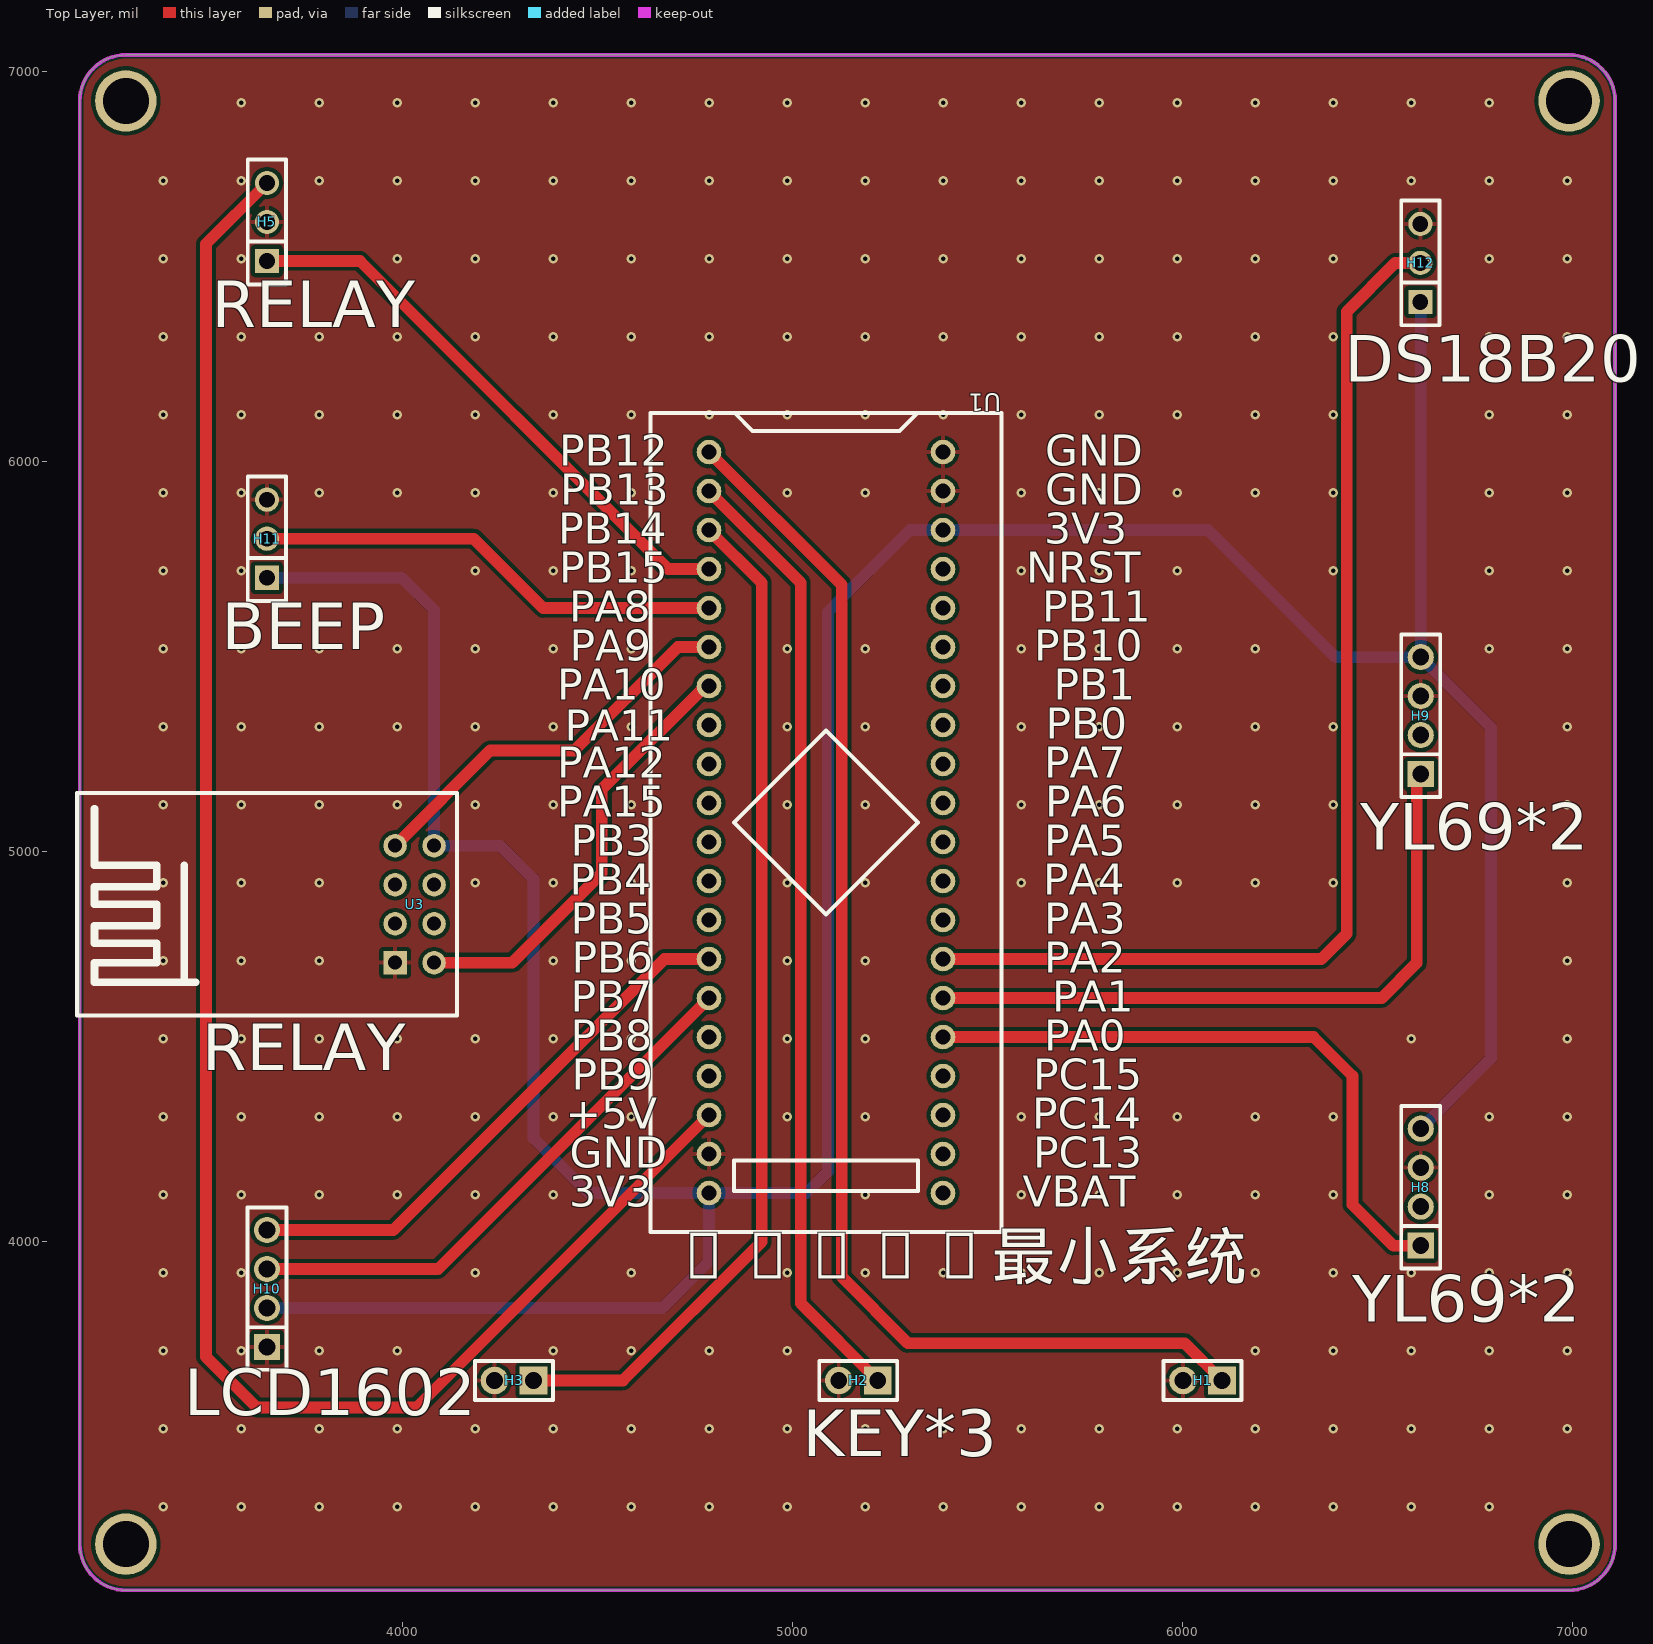
[diagram p0: Top Layer view]
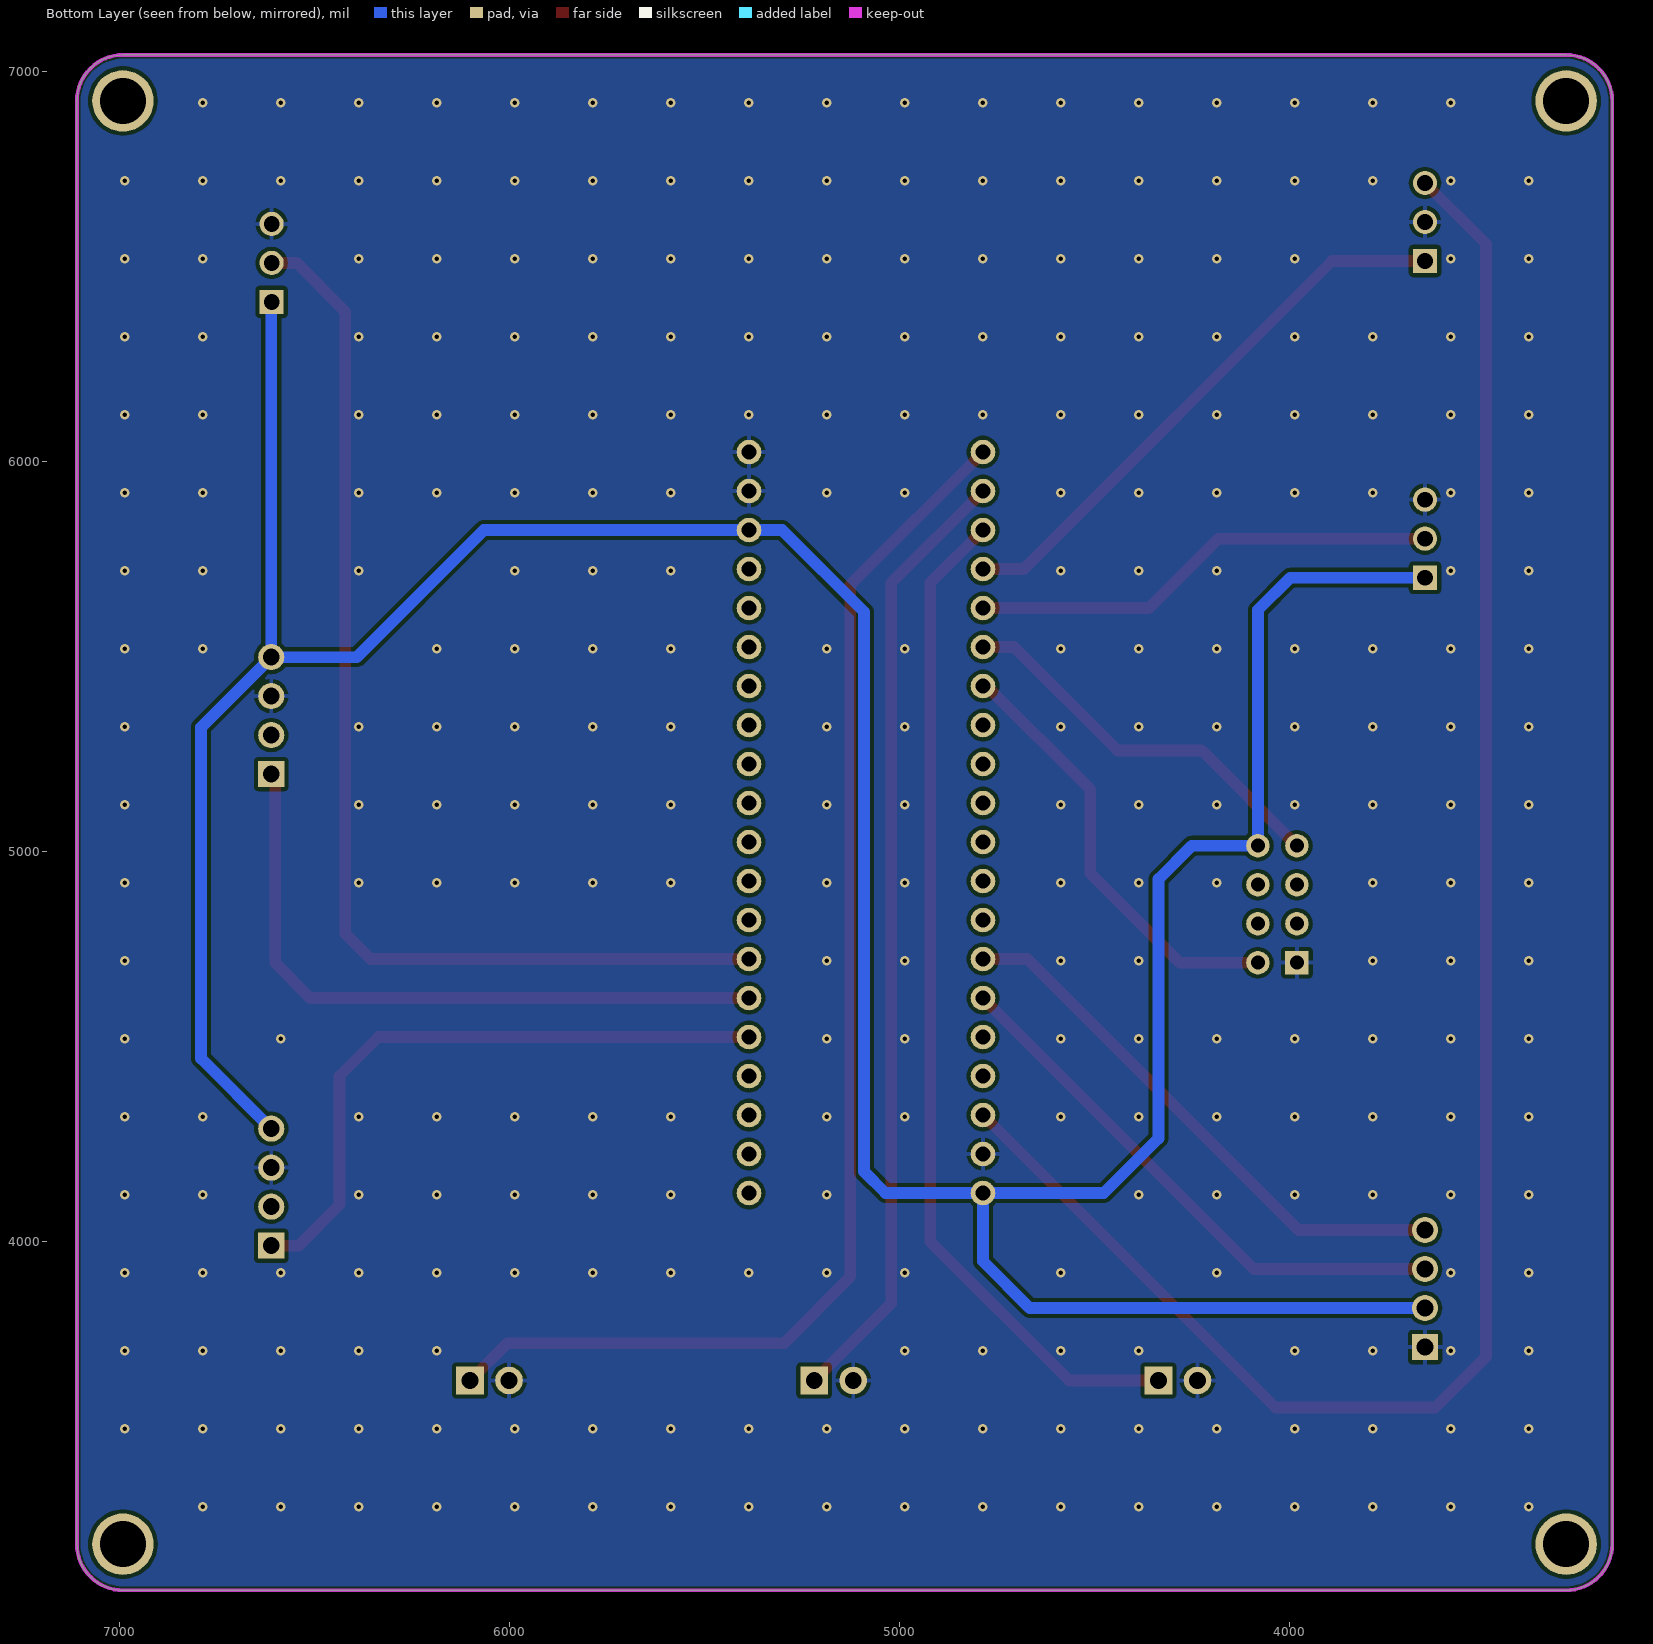
[diagram p1: Bottom Layer view, seen from below]
# Altium PCB MISC51268.pcbdoc
Units mil, origin at the board's own origin, x right, y up, seen from the top; angles counter-clockwise.
Board outline 3937.01 x 3937.01 mil, 2 copper layers (Top Layer, Bottom Layer), stack 62.206 mil thick; 11 components, 37 nets, 79 pads, 289 vias.

## Layer stack, top to bottom
Top Solder Mask Layer: solder mask 0.394, Dk 3.3
Top Layer: signal copper 1.379
Dielectric1: surface 59.449, FR4, Dk 4.5
Bottom Layer: signal copper 1.378
Bottom Solder Mask Layer: solder mask 0.394, Dk 3.3

## Board outline
6990.39,3106.5 ccw(c6990.39,3224.61) 7108.5,3224.61 7108.5,6925.39 ccw(c6990.39,6925.39) 6990.39,7043.5 3289.61,7043.5 ccw(c3289.61,6925.39) 3171.5,6925.39 3171.5,3224.61 ccw(c3289.61,3224.61) 3289.61,3106.5

## Design rules (kind name [scope] priority, off if disabled: settings)
BoardOutlineClearance copperThickness2oz_1 [All] p2 off: genericclearance=7.99 ignorepadtopadclearanceinfootprint=FALSE except(0: Arc-SplitContinuation Track-SplitContinuation SMDPad-SplitContinuation THPad-SplitContinuation Via-SplitContinuation Fill-SplitContinuation Region-SplitContinuation Poly-SplitContinuation Text-SplitContinuation Hole-SplitContinuation; 5.98: Arc-CutoutEdge Track-CutoutEdge SMDPad-CutoutEdge THPad-CutoutEdge Via-CutoutEdge Text-CutoutEdge; 6.89: Hole-OutlineEdge Hole-CutoutEdge; 10: Poly-OutlineEdge Poly-CutoutEdge; 11.81: Arc-OutlineEdge Track-OutlineEdge SMDPad-OutlineEdge THPad-OutlineEdge Via-OutlineEdge Fill-OutlineEdge Region-OutlineEdge Text-OutlineEdge Fill-CutoutEdge Region-CutoutEdge)
BoardOutlineClearance Plane_innerPlane_1 [All] p4 off: genericclearance=4.02 ignorepadtopadclearanceinfootprint=FALSE except(0: Arc-SplitContinuation Track-SplitContinuation SMDPad-SplitContinuation THPad-SplitContinuation Via-SplitContinuation Fill-SplitContinuation Region-SplitContinuation Poly-SplitContinuation Text-SplitContinuation Hole-SplitContinuation; 5.98: Arc-CutoutEdge Track-CutoutEdge SMDPad-CutoutEdge THPad-CutoutEdge Via-CutoutEdge Text-CutoutEdge; 6.89: Hole-OutlineEdge Hole-CutoutEdge; 10: Poly-OutlineEdge Poly-CutoutEdge; 11.81: Arc-OutlineEdge Track-OutlineEdge SMDPad-OutlineEdge THPad-OutlineEdge Via-OutlineEdge Fill-OutlineEdge Region-OutlineEdge Text-OutlineEdge Fill-CutoutEdge Region-CutoutEdge)
BoardOutlineClearance Copper_copperRegion_1 [All] p6 off: genericclearance=4.02 ignorepadtopadclearanceinfootprint=FALSE except(0: Arc-SplitContinuation Track-SplitContinuation SMDPad-SplitContinuation THPad-SplitContinuation Via-SplitContinuation Fill-SplitContinuation Region-SplitContinuation Poly-SplitContinuation Text-SplitContinuation Hole-SplitContinuation; 5.98: Arc-CutoutEdge Track-CutoutEdge SMDPad-CutoutEdge THPad-CutoutEdge Via-CutoutEdge Text-CutoutEdge; 6.89: Hole-OutlineEdge Hole-CutoutEdge; 10: Poly-OutlineEdge Poly-CutoutEdge; 11.81: Arc-OutlineEdge Track-OutlineEdge SMDPad-OutlineEdge THPad-OutlineEdge Via-OutlineEdge Fill-OutlineEdge Region-OutlineEdge Text-OutlineEdge Fill-CutoutEdge Region-CutoutEdge)
BoardOutlineClearance copperThickness1oz_1 [All] p8: genericclearance=4.02 ignorepadtopadclearanceinfootprint=FALSE except(0: Arc-SplitContinuation Track-SplitContinuation SMDPad-SplitContinuation THPad-SplitContinuation Via-SplitContinuation Fill-SplitContinuation Region-SplitContinuation Poly-SplitContinuation Text-SplitContinuation Hole-SplitContinuation; 5.98: Arc-CutoutEdge Track-CutoutEdge SMDPad-CutoutEdge THPad-CutoutEdge Via-CutoutEdge Text-CutoutEdge; 6.89: Hole-OutlineEdge Hole-CutoutEdge; 10: Poly-OutlineEdge Poly-CutoutEdge; 11.81: Arc-OutlineEdge Track-OutlineEdge SMDPad-OutlineEdge THPad-OutlineEdge Via-OutlineEdge Fill-OutlineEdge Region-OutlineEdge Text-OutlineEdge Fill-CutoutEdge Region-CutoutEdge)
Clearance copperThickness2oz [All] p1 off: gap=7.99 ignorepadtopadclearanceinfootprint=FALSE except(5.98: SMDPad-Track SMDPad-SMDPad THPad-Track SMDPad-THPad THPad-THPad Track-Via SMDPad-Via THPad-Via Via-Via Fill-SMDPad Region-SMDPad Fill-THPad Region-THPad Fill-Via Region-Via Fill-Fill Fill-Region Region-Region Arc-Track Arc-SMDPad Arc-THPad Arc-Via Fill-Arc Region-Arc Arc-Arc Text-Track SMDPad-Text Text-THPad Text-Via Fill-Text Region-Text Arc-Text Text-Text; 6.89: Hole-Track Hole-SMDPad Hole-THPad Hole-Via Fill-Hole Region-Hole Hole-Arc Hole-Text; 10: Poly-Track Poly-SMDPad Poly-THPad Poly-Via Poly-Fill Poly-Region Poly-Poly Poly-Arc Poly-Text Poly-Hole; 11.81: Fill-Track Region-Track)
Clearance Plane_innerPlane [All] p3 off: gap=4.02 ignorepadtopadclearanceinfootprint=FALSE except(5.98: SMDPad-Track SMDPad-SMDPad THPad-Track SMDPad-THPad THPad-THPad Track-Via SMDPad-Via THPad-Via Via-Via Fill-SMDPad Region-SMDPad Fill-THPad Region-THPad Fill-Via Region-Via Fill-Fill Fill-Region Region-Region Arc-Track Arc-SMDPad Arc-THPad Arc-Via Fill-Arc Region-Arc Arc-Arc Text-Track SMDPad-Text Text-THPad Text-Via Fill-Text Region-Text Arc-Text Text-Text; 6.89: Hole-Track Hole-SMDPad Hole-THPad Hole-Via Fill-Hole Region-Hole Hole-Arc Hole-Text; 10: Poly-Track Poly-SMDPad Poly-THPad Poly-Via Poly-Fill Poly-Region Poly-Poly Poly-Arc Poly-Text Poly-Hole; 11.81: Fill-Track Region-Track)
Clearance Copper_copperRegion [All] p5 off: gap=4.02 ignorepadtopadclearanceinfootprint=FALSE except(5.98: SMDPad-Track SMDPad-SMDPad THPad-Track SMDPad-THPad THPad-THPad Track-Via SMDPad-Via THPad-Via Via-Via Fill-SMDPad Region-SMDPad Fill-THPad Region-THPad Fill-Via Region-Via Fill-Fill Fill-Region Region-Region Arc-Track Arc-SMDPad Arc-THPad Arc-Via Fill-Arc Region-Arc Arc-Arc Text-Track SMDPad-Text Text-THPad Text-Via Fill-Text Region-Text Arc-Text Text-Text; 6.89: Hole-Track Hole-SMDPad Hole-THPad Hole-Via Fill-Hole Region-Hole Hole-Arc Hole-Text; 10: Poly-Track Poly-SMDPad Poly-THPad Poly-Via Poly-Fill Poly-Region Poly-Poly Poly-Arc Poly-Text Poly-Hole; 11.81: Fill-Track Region-Track)
Clearance copperThickness1oz [All] p7: gap=4.02 ignorepadtopadclearanceinfootprint=FALSE except(5.98: SMDPad-Track SMDPad-SMDPad THPad-Track SMDPad-THPad THPad-THPad Track-Via SMDPad-Via THPad-Via Via-Via Fill-SMDPad Region-SMDPad Fill-THPad Region-THPad Fill-Via Region-Via Fill-Fill Fill-Region Region-Region Arc-Track Arc-SMDPad Arc-THPad Arc-Via Fill-Arc Region-Arc Arc-Arc Text-Track SMDPad-Text Text-THPad Text-Via Fill-Text Region-Text Arc-Text Text-Text; 6.89: Hole-Track Hole-SMDPad Hole-THPad Hole-Via Fill-Hole Region-Hole Hole-Arc Hole-Text; 10: Poly-Track Poly-SMDPad Poly-THPad Poly-Via Poly-Fill Poly-Region Poly-Poly Poly-Arc Poly-Text Poly-Hole; 11.81: Fill-Track Region-Track)
DiffPairsRouting differentialPair [All] p1: maxlimit=6 minlimit=6 mostfreqgap=6 toplayer_minwidth=5 toplayer_prefwidth=10 toplayer_maxwidth=100 toplayer_mingap=6 toplayer_prefgap=6 toplayer_maxgap=6 bottomlayer_minwidth=5 bottomlayer_prefwidth=10 bottomlayer_maxwidth=100 bottomlayer_mingap=6 bottomlayer_prefgap=6 bottomlayer_maxgap=6 maxuncoupledlength=10
HoleToHoleClearance otherClearance [All] p1: gap=11.81 allowstackedmicrovias=TRUE
Length netLength [All] p1: minlimit=0 maxlimit=0
PasteMaskExpansion pasteMaskExpansion [All] p1: expansion=0
PlaneConnect innerPlane [All] p1: planeconnectstyle=Relief reliefexpansion=20 reliefentries=4 reliefconductorwidth=10 reliefairgap=10
PolygonConnect copperRegion [All] p1: connectstyle=Relief reliefconductorwidth=10 reliefentries=4 polygonreliefangle="90 Angle" airgapwidth=10 via.connectstyle=Relief via.reliefconductorwidth=10 via.reliefentries=4 via.polygonreliefangle="90 Angle" via.airgapwidth=10
RoutingVias viaSize [All] p1: holewidth=12.01 width=24.02 viastyle="Through Hole" minholewidth=11.81 minwidth=19.68 maxholewidth=248.03 maxwidth=393.7
SolderMaskExpansion solderMaskExpansion [IsVia] p1: expansion=-1000 istentingtop=TRUE
SolderMaskExpansion solderMaskExpansion [All] p2: expansion=2.01 istentingtop=FALSE
Width copperThickness2oz_2 [All] p1 off: maxlimit=100 minlimit=8 preferedwidth=10
Width copperThickness1oz_2 [All] p2: maxlimit=100 minlimit=5 preferedwidth=30

## Components (designator, comment, footprint, x,y, rotation, side; value= is the part's Value field where it differs from the comment)
H1 "" HDR-TH_2P-P2.54-V-M-1 6050.45,3644.31 r180 top
H2 "" HDR-TH_2P-P2.54-V-M-1 5167.73,3644.31 r180 top
H3 "" HDR-TH_2P-P2.54-V-M-1 4285,3644.31 r180 top
H5 "" HDR-TH_3P-P2.54-V-F 3651.55,6615 r90 top
H8 "" HDR-TH_4P-P2.54-V-F 6610,4140 r90 top
H9 "" HDR-TH_4P-P2.54-V-F 6610,5349.21 r90 top
H10 "" HDR-TH_4P-P2.54-V-F 3651.55,3880 r90 top
H11 "" HDR-TH_3P-P2.54-V-F 3651.55,5802.91 r90 top
H12 "" HDR-TH_3P-P2.54-V-F 6609.21,6510 r90 top
U1 "STM32F103C8T6-Card" CONN-TH_L53.3-W22.9_STM32F103C8T6-CARD 5085,5075 r270 top
U3 "ESP8266-01S" WIFIM-TH_ESP8266-01S 4030,4865.67 r90 top

## Footprints (in the part's own frame and the unit in brackets; to place one, negate y for a bottom-side part, rotate by r counter-clockwise, add the part's x,y. Pads: shape width x height; smd on the part's side, far side on the other; paste and mask are expansions set on the pad)
CONN-TH_L53.3-W22.9_STM32F103C8T6-CARD [mm]
  round 1.6 hole 1: 1(-24.13,-7.62) 2(-21.59,-7.62) 3(-19.05,-7.62) 4(-16.51,-7.62) 5(-13.97,-7.62) 6(-11.43,-7.62) 7(-8.89,-7.62) 8(-6.35,-7.62) 9(-3.81,-7.62) 10(-1.27,-7.62) 11(1.27,-7.62) 12(3.81,-7.62) 13(6.35,-7.62) 14(8.89,-7.62) 15(11.43,-7.62) 16(13.97,-7.62) 17(16.51,-7.62) 18(19.05,-7.62) 19(21.59,-7.62) 20(24.13,-7.62) 21(24.13,7.62) 22(21.59,7.62) 23(19.05,7.62) 24(16.51,7.62) 25(13.97,7.62) 26(11.43,7.62) 27(8.89,7.62) 28(6.35,7.62) 29(3.81,7.62) 30(1.27,7.62) 31(-1.27,7.62) 32(-3.81,7.62) 33(-6.35,7.62) 34(-8.89,7.62) 35(-11.43,7.62) 36(-13.97,7.62) 37(-16.51,7.62) 38(-19.05,7.62) 39(-21.59,7.62) 40(-24.13,7.62)
  silkscreen extent -26.67,-11.43 26.67,11.43
HDR-TH_2P-P2.54-V-M-1 [mm]
  rect 1.8x1.8 hole 1.1: 1(-1.27,0)
  round 1.8 hole 1.1: 2(1.27,0)
  silkscreen extent -2.54,-1.27 2.54,1.27
HDR-TH_3P-P2.54-V-F [mil]
  rect 62x62 hole 40.16: 1(-100,0)
  round 62 hole 40.16: 2(0,0) 3(100,0)
  silkscreen extent -160,-49 160,49
HDR-TH_4P-P2.54-V-F [mm]
  rect 1.7x1.7 hole 1.1: 1(-3.81,0)
  round 1.7 hole 1.1: 2(-1.27,0) 3(1.27,0) 4(3.81,0)
  silkscreen extent -5.29,-1.27 5.29,1.27
WIFIM-TH_ESP8266-01S [mil]
  rect 60x60 hole 36 paste+0 mask+1.97: 1(-150,50)
  round 60 hole 36 paste+0 mask+1.97: 2(-50,50) 3(50,50) 4(150,50) 5(-150,-50) 6(-50,-50) 7(50,-50) 8(150,-50)
  silkscreen extent -285,-109 285,866

## Free pads (board coordinates)
  round 157.48 hole 118.11: 1(3289.61,6925.39) 1(3289.61,3224.61) 1(6990.39,6925.39) 1(6990.39,3224.61)

## Via types
v1: diameter 24.02, hole 12, Top Layer to Bottom Layer, 289 vias

## Nets (pads, with @x,y where several pads share a name; then routed paths per layer and width w, separated by ;. In a path a pad name is that pad's centre, name@x,y a point inside that pad or via, vN(x,y) a via of type N, cw(c..) or ccw(c..) an arc to the next point about the centre after c; other vN are vias at no path point)
+5V: H5.3 U1.18 | length 4729.4
  Top Layer w30: H5.3 3495,6558.44 3495,3705 3625,3575 4035,3575 U1.18
GND: H1.2 H2.2 H3.2 H5.2 H8.3 H9.3 H10.1 H11.3 H12.3 U1.19 U1.39 U1.40 U3.1
  other v1: 3385.6,3320.6 3585.6,3320.6 3785.6,3320.6 3985.6,3320.6 4185.6,3320.6 4385.6,3320.6 4585.6,3320.6 4785.6,3320.6 4985.6,3320.6 5185.6,3320.6 5385.6,3320.6 5585.6,3320.6 5785.6,3320.6 5985.6,3320.6 6185.6,3320.6 6385.6,3320.6 6585.6,3320.6 6785.6,3320.6 3385.6,3520.6 3585.6,3520.6 3785.6,3520.6 3985.6,3520.6 4185.6,3520.6 4385.6,3520.6 4585.6,3520.6 4785.6,3520.6 4985.6,3520.6 5185.6,3520.6 5385.6,3520.6 5585.6,3520.6 5785.6,3520.6 5985.6,3520.6 6185.6,3520.6 6385.6,3520.6 6585.6,3520.6 6785.6,3520.6 6985.6,3520.6 3385.6,3720.6 3585.6,3720.6 3785.6,3720.6 3985.6,3720.6 4385.6,3720.6 4585.6,3720.6 4785.6,3720.6 4985.6,3720.6 6185.6,3720.6 6385.6,3720.6 6585.6,3720.6 6785.6,3720.6 6985.6,3720.6 3385.6,3920.6 3585.6,3920.6 4185.6,3920.6 4585.6,3920.6 4985.6,3920.6 5185.6,3920.6 5385.6,3920.6 5585.6,3920.6 5785.6,3920.6 5985.6,3920.6 6185.6,3920.6 6385.6,3920.6 6585.6,3920.6 6785.6,3920.6 6985.6,3920.6 3385.6,4120.6 3585.6,4120.6 3785.6,4120.6 3985.6,4120.6 4185.6,4120.6 4385.6,4120.6 5185.6,4120.6 5585.6,4120.6 5785.6,4120.6 5985.6,4120.6 6185.6,4120.6 6385.6,4120.6 6785.6,4120.6 6985.6,4120.6 3385.6,4320.6 3585.6,4320.6 3785.6,4320.6 3985.6,4320.6 4185.6,4320.6 4385.6,4320.6 4585.6,4320.6 4985.6,4320.6 5185.6,4320.6 5585.6,4320.6 5785.6,4320.6 5985.6,4320.6 6185.6,4320.6 6385.6,4320.6 6785.6,4320.6 6985.6,4320.6 3385.6,4520.6 3585.6,4520.6 3785.6,4520.6 3985.6,4520.6 4185.6,4520.6 4385.6,4520.6 4585.6,4520.6 4985.6,4520.6 5185.6,4520.6 6585.6,4520.6 6985.6,4520.6 3385.6,4720.6 3585.6,4720.6 3785.6,4720.6 4385.6,4720.6 4585.6,4720.6 4985.6,4720.6 5185.6,4720.6 6985.6,4720.6 3385.6,4920.6 3585.6,4920.6 3785.6,4920.6 4185.6,4920.6 4385.6,4920.6 4585.6,4920.6 4985.6,4920.6 5185.6,4920.6 5585.6,4920.6 5785.6,4920.6 5985.6,4920.6 6185.6,4920.6 6385.6,4920.6 6985.6,4920.6 3385.6,5120.6 3585.6,5120.6 3785.6,5120.6 3985.6,5120.6 4185.6,5120.6 4385.6,5120.6 4585.6,5120.6 4985.6,5120.6 5185.6,5120.6 5585.6,5120.6 5785.6,5120.6 5985.6,5120.6 6185.6,5120.6 6385.6,5120.6 6985.6,5120.6 3385.6,5320.6 3585.6,5320.6 3785.6,5320.6 3985.6,5320.6 4185.6,5320.6 4385.6,5320.6 4585.6,5320.6 4985.6,5320.6 5185.6,5320.6 5585.6,5320.6 5785.6,5320.6 5985.6,5320.6 6185.6,5320.6 6385.6,5320.6 6985.6,5320.6 3385.6,5520.6 3585.6,5520.6 3785.6,5520.6 3985.6,5520.6 4185.6,5520.6 4385.6,5520.6 4585.6,5520.6 4985.6,5520.6 5185.6,5520.6 5585.6,5520.6 5785.6,5520.6 5985.6,5520.6 6185.6,5520.6 6785.6,5520.6 6985.6,5520.6 3385.6,5720.6 3585.6,5720.6 4185.6,5720.6 4385.6,5720.6 4585.6,5720.6 5585.6,5720.6 5785.6,5720.6 5985.6,5720.6 6385.6,5720.6 6785.6,5720.6 6985.6,5720.6 3385.6,5920.6 3585.6,5920.6 3785.6,5920.6 3985.6,5920.6 4185.6,5920.6 4385.6,5920.6 4585.6,5920.6 4985.6,5920.6 5185.6,5920.6 5585.6,5920.6 5785.6,5920.6 5985.6,5920.6 6185.6,5920.6 6385.6,5920.6 6785.6,5920.6 6985.6,5920.6 3385.6,6120.6 3585.6,6120.6 3785.6,6120.6 3985.6,6120.6 4185.6,6120.6 4385.6,6120.6 4585.6,6120.6 4785.6,6120.6 4985.6,6120.6 5185.6,6120.6 5385.6,6120.6 5585.6,6120.6 5785.6,6120.6 5985.6,6120.6 6185.6,6120.6 6385.6,6120.6 6785.6,6120.6 6985.6,6120.6 3385.6,6320.6 3585.6,6320.6 3785.6,6320.6 3985.6,6320.6 4185.6,6320.6 4385.6,6320.6 4585.6,6320.6 4785.6,6320.6 4985.6,6320.6 5185.6,6320.6 5385.6,6320.6 5585.6,6320.6 5785.6,6320.6 5985.6,6320.6 6185.6,6320.6 6385.6,6320.6 6785.6,6320.6 6985.6,6320.6 3385.6,6520.6 3585.6,6520.6 3985.6,6520.6 4185.6,6520.6 4385.6,6520.6 4585.6,6520.6 4785.6,6520.6 4985.6,6520.6 5185.6,6520.6 5385.6,6520.6 5585.6,6520.6 5785.6,6520.6 5985.6,6520.6 6185.6,6520.6 6385.6,6520.6 6785.6,6520.6 6985.6,6520.6 3385.6,6720.6 3585.6,6720.6 3785.6,6720.6 3985.6,6720.6 4185.6,6720.6 4385.6,6720.6 4585.6,6720.6 4785.6,6720.6 4985.6,6720.6 5185.6,6720.6 5385.6,6720.6 5585.6,6720.6 5785.6,6720.6 5985.6,6720.6 6185.6,6720.6 6385.6,6720.6 6585.6,6720.6 6785.6,6720.6 6985.6,6720.6 3585.6,6920.6 3785.6,6920.6 3985.6,6920.6 4185.6,6920.6 4385.6,6920.6 4585.6,6920.6 4785.6,6920.6 4985.6,6920.6 5185.6,6920.6 5385.6,6920.6 5585.6,6920.6 5785.6,6920.6 5985.6,6920.6 6185.6,6920.6 6385.6,6920.6 6585.6,6920.6 6785.6,6920.6
NRST: U1.37
PA0: H8.1 U1.25 | length 1639.9
  Top Layer w30: U1.25 6335,4525 6435,4425 6435,4095 6540,3990 H8.1
PA1: H9.1 U1.26 | length 1740.6
  Top Layer w30: U1.26 6510,4625 6600,4715 6600,5189.21 H9.1
PA2: H12.2 U1.27 | length 2897.9
  Top Layer w30: U1.27 6355,4725 6420,4790 6420,6385 6545,6510 H12.2
PA3: U1.28
PA4: U1.29
PA5: U1.30
PA6: U1.31
PA7: U1.32
PA8: H11.2 U1.5 | length 1207.1
  Top Layer w30: H11.2 4182.09,5802.91 4360,5625 U1.5
PA9: U1.6 U3.4 | length 1016
  Top Layer w30: U3.4 4224.33,5260 4440,5260 4705,5525 U1.6
PA10: U1.7 U3.5 | length 1124.8
  Top Layer w30: U3.5 4280.67,4715.67 4510,4945 4510,5160 4775,5425 U1.7
PA11: U1.8
PA12: U1.9
PA15: U1.10
PB0: U1.33
PB1: U1.34
PB3: U1.11
PB4: U1.12
PB5: U1.13
PB6: H10.4 U1.14 | length 1421.3
  Top Layer w30: H10.4 3975,4030 4670,4725 U1.14
PB7: H10.3 U1.15 | length 1421.3
  Top Layer w30: H10.3 4090,3930 U1.15
PB8: U1.16
PB9: U1.17
PB10: U1.35
PB11: U1.36
PB12: H1.1 U1.1 | length 3341.3
  Top Layer w30: U1.1 5125,5685 5125,3910 5295,3740 6004.76,3740 H1.1
PB13: H2.1 U1.2 | length 2459.9
  Top Layer w30: U1.2 5020,5690 5020,3842.04 H2.1
PB14: H3.1 U1.3 | length 2613.2
  Top Layer w30: H3.1 4564.31,3644.31 4920,4000 4920,5690 U1.3
PB15: H5.1 U1.4 | length 1460.7
  Top Layer w30: H5.1 3890,6515 4680,5725 U1.4
PC13: U1.22
PC14: U1.23
PC15: U1.24
VBAT: U1.21
VCC: H8.4 H9.4 H10.2 H11.1 H12.1 U1.20 U1.38 U3.8 | length 9662.9
  Bottom Layer w30: H10.2 4665,3830 4785,3950 U1.20 ; H11.1 3997.09,5702.91 4080,5620 U3.8 4249.33,5015.67 4335,4930 4335,4265 4475,4125 U1.20 ; H12.1 6610,6409.21 H9.4 ; H8.4 6790,4470 6790,5319.21 H9.4 ; U1.20 5035,4125 5090,4180 5090,5615 5300,5825 U1.38 6065,5825 6390.79,5499.21 H9.4
pads on no net: H8.2 H9.2 U3.2 U3.3 U3.6 U3.7

## Polygon pours and split planes (outlines as drawn)
GND on Bottom Layer (solid, remove dead copper, pour order 2): 3100,7165 3100,3000 7275,3000 7275,7165
GND on Top Layer (solid, remove dead copper, pour order 0): 3000,7145 3000,3075 7385,3075 7385,7145

## Keep-outs
Board Outline Layer:
  the board outline again, w10

## Silkscreen, mask and mechanical layers (free items; w line width, h text height)
Top Silkscreen Layer:
  text "RELAY" at 3510,6345 h120
  text "DS18B20" at 6415,6205 h120
  text "PB12" at 4400.64,5990 h80
  text "GND" at 5646.65,5990 h80
  text "PB13" at 4403.85,5890 h80
  text "GND" at 5646.65,5890 h80
  text "PB14" at 4398.34,5790 h80
  text "3V3" at 5644.45,5790 h80
  text "PB15" at 4400.64,5690 h80
  text "NRST" at 5598.65,5690 h80
  text "PA8" at 4426.24,5590 h80
  text "PB11" at 5639.05,5590 h80
  text "BEEP" at 3535,5520 h120
  text "PA9" at 4428.44,5490 h80
  text "PB10" at 5618.85,5490 h80
  text "PA10" at 4396.14,5390 h80
  text "PB1" at 5669.15,5390 h80
  text "PB0" at 5648.95,5290 h80
  text "PA11" at 4414.55,5285 h80
  text "PA12" at 4396.14,5190 h80
  text "PA7" at 5644.45,5190 h80
  text "PA15" at 4396.14,5090 h80
  text "PA6" at 5646.65,5090 h80
  text "YL69*2" at 6455,5005 h120
  text "PB3" at 4430.74,4990 h80
  text "PA5" at 5644.45,4990 h80
  text "PB4" at 4428.44,4890 h80
  text "PA4" at 5642.15,4890 h80
  text "PB5" at 4430.74,4790 h80
  text "PA3" at 5644.45,4790 h80
  text "PB6" at 4432.94,4690 h80
  text "PA2" at 5644.45,4690 h80
  text "PB7" at 4430.74,4590 h80
  text "PA1" at 5664.65,4590 h80
  text "PB8" at 4430.74,4490 h80
  text "PA0" at 5644.45,4490 h80
  text "RELAY" at 3485,4440 h120
  text "PB9" at 4432.94,4390 h80
  text "PC15" at 5616.55,4390 h80
  text "+5V" at 4417.24,4290 h80
  text "PC14" at 5614.25,4290 h80
  text "GND" at 4428.44,4190 h80
  text "PC13" at 5616.55,4190 h80
  text "3V3" at 4426.24,4090 h80
  text "VBAT" at 5589.65,4090 h80
  text "STM32最小系统" at 4690,3905 h120
  text "YL69*2" at 6435,3795 h120
  text "LCD1602" at 3440,3555 h120
  text "KEY*3" at 5025,3450 h120